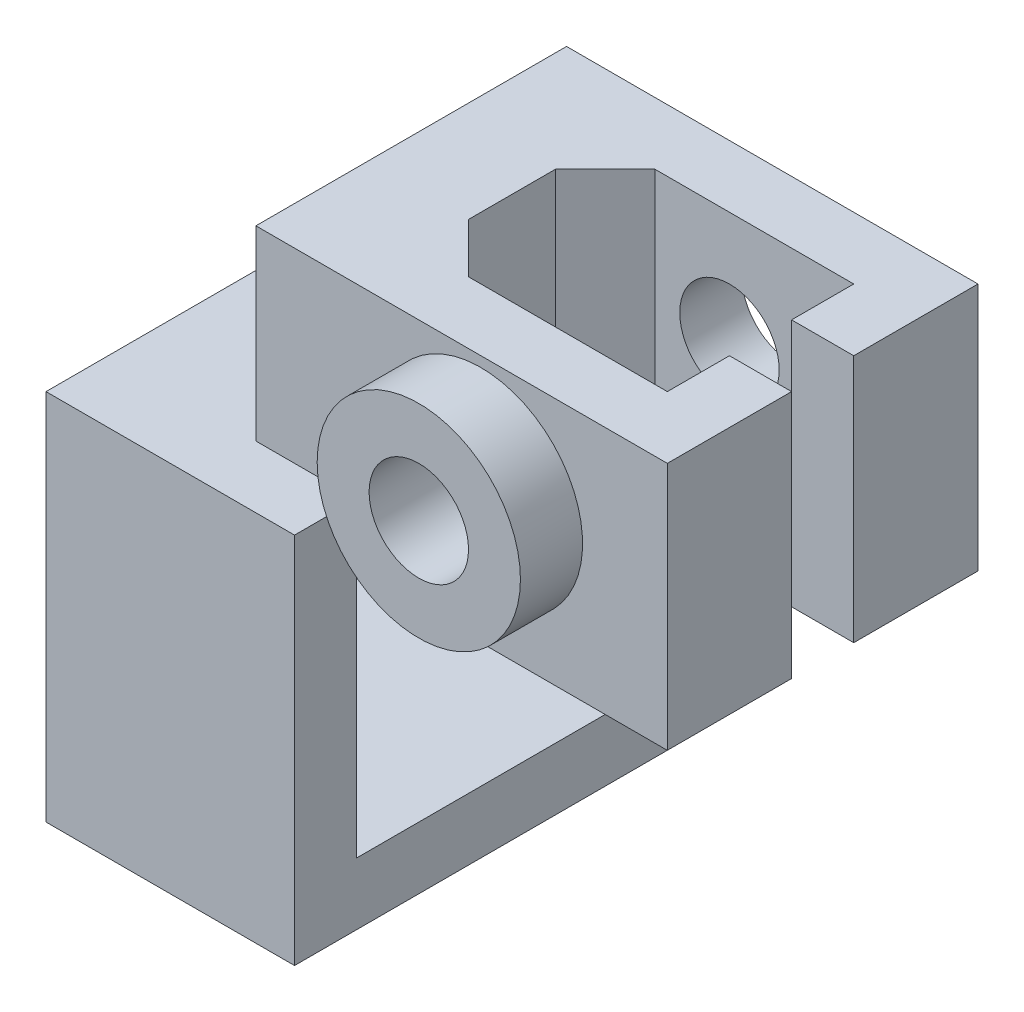
from build123d import *

# Parameters (mm, degrees)
SKETCH1_W           = 40
SKETCH1_H           = 50
BOSS_EXTRUDE1_DEPTH = 10
BOSS_EXTRUDE2_DEPTH = 10
BOSS_EXTRUDE3_DEPTH = 40
BOSS_EXTRUDE4_DEPTH = 30
SKETCH5_R           = 8
CUT_EXTRUDE1_DEPTH  = 50
SKETCH6_R           = 16.35789331
SKETCH6_R_2         = 8
BOSS_EXTRUDE5_DEPTH = 10


with BuildPart() as part:
    # Sketch1 → Boss-Extrude1 (new body)
    with BuildSketch(Plane(origin=(0, 0, 0), x_dir=(1, 0, 0), z_dir=(0, 1, 0))):
        Rectangle(SKETCH1_W, SKETCH1_H)
    extrude(amount=BOSS_EXTRUDE1_DEPTH)

    # Sketch2 → Boss-Extrude2 (add)
    with BuildSketch(Plane(origin=(0, 10, 0), x_dir=(1, 0, 0), z_dir=(0, 1, 0))):
        Polygon((28, -15), (60, -15), (60, -5), (70, -5), (70, -25), (20, -25), (20, -15), (20, -7), align=None)
        Polygon((20, 25), (70, 25), (70, 5), (60, 5), (60, 15), (28, 15), (20, 7), (20, 15), align=None)
    extrude(amount=-BOSS_EXTRUDE2_DEPTH)

    # Sketch3 → Boss-Extrude3 (add)
    with BuildSketch(Plane.ZY.offset(20)):
        Polygon((-25, 10), (-35, 10), (-35, -50), (35, -50), (35, 10), (25, 10), (25, 0), (25, -40), (-25, -40), (-25, 0), align=None)
    extrude(amount=-BOSS_EXTRUDE3_DEPTH)

    # Sketch4 → Boss-Extrude4 (add)
    with BuildSketch(Plane(origin=(0, 10, 0), x_dir=(1, 0, 0), z_dir=(0, 1, 0))):
        Polygon((20, 7), (28, 15), (60, 15), (60, 5), (70, 5), (70, 25), (3.779860002, 25), (3.779860002, -25), (70, -25), (70, -5), (60, -5), (60, -15), (28, -15), (20, -7), align=None)
    extrude(amount=BOSS_EXTRUDE4_DEPTH)

    # Sketch5 → Cut-Extrude1 (cut)
    with BuildSketch(Plane(origin=(0, 0, -25), x_dir=(-1, 0, 0), z_dir=(0, 0, -1))):
        with Locations((-40, 22)):
            Circle(SKETCH5_R)
    extrude(amount=-CUT_EXTRUDE1_DEPTH, mode=Mode.SUBTRACT)

    # Sketch6 → Boss-Extrude5 (add)
    with BuildSketch(Plane.XY.offset(25)):
        with Locations(Location((40, 22, 0), (0, 0, 180))):
            Circle(SKETCH6_R)
        with Locations(Location((40, 22, 0), (0, 0, 180))):
            Circle(SKETCH6_R_2, mode=Mode.SUBTRACT)
    extrude(amount=BOSS_EXTRUDE5_DEPTH)


solid = part.part
